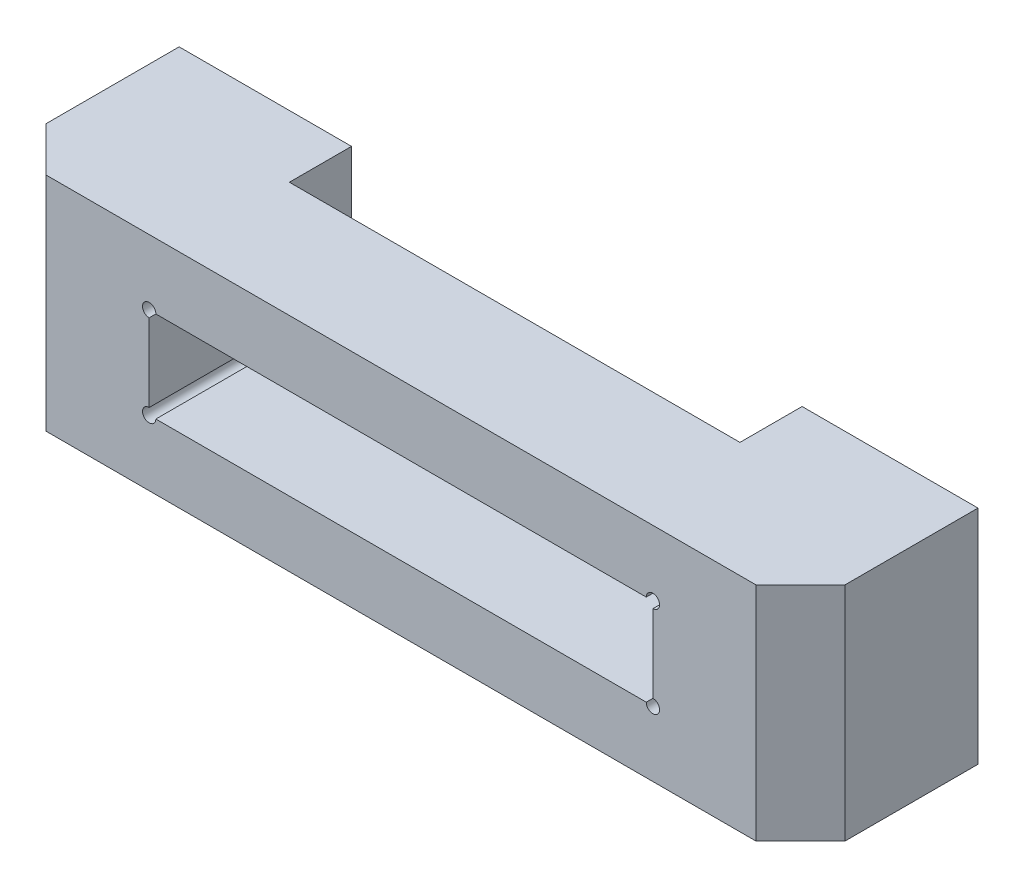
SolidWorks part; units mm, degrees
ref_plane "Front Plane" through (0, 0, 0) normal (0, 0, 1) x (1, 0, 0)
ref_plane "Top Plane" through (0, 0, 0) normal (0, 1, 0) x (1, 0, 0)
ref_plane "Right Plane" through (0, 0, 0) normal (1, 0, 0) x (0, 0, -1)
sketch "Sketch1" plane through (0, 0, 0) normal (0, 0, 1) x (1, 0, 0)
  line L0 (-90, 25) -> (90, -25) construction
  line L1 (-90, 25) -> (90, 25)
  line L2 (-90, 25) -> (-90, -25)
  line L3 (-90, -25) -> (90, -25)
  line L4 (90, 25) -> (90, -25)
  dimension "D1" = 180
  dimension "D2" = 50
extrude "Boss-Extrude1" add sketch "Sketch1" along normal blind 40
sketch "Sketch2" plane through (0, 0, 40) normal (0, 0, 1) x (1, 0, 0)
  line L1 (-56.75, 10.25) -> (56.75, 10.25)
  line L2 (-56.75, 10.25) -> (-56.75, -10.25)
  line L3 (-56.75, -10.25) -> (56.75, -10.25)
  line L4 (56.75, 10.25) -> (56.75, -10.25)
  line L5 (-56.75, 10.25) -> (56.75, -10.25) construction
  line L6 (-56.75, -10.25) -> (56.75, 10.25) construction
  point P0 (0, 0)
  dimension "D1" = 113.5
  dimension "D2" = 20.5
extrude "Cut-Extrude1" cut sketch "Sketch2" against normal through all
sketch "Sketch3" plane through (0, 0, 40) normal (0, 0, 1) x (1, 0, 0)
  circle A0 centre (-56.75, 10.25) radius 1.5
  circle A1 centre (-56.75, -10.25) radius 1.5
  circle A2 centre (56.75, 10.25) radius 1.5
  circle A3 centre (56.75, -10.25) radius 1.5
  dimension "D1" = 3
extrude "Cut-Extrude2" cut sketch "Sketch3" against normal through all
sketch "Sketch4" plane through (0, 25, 0) normal (0, 1, 0) x (1, 0, 0)
  line L0 (90, 0) -> (-90, 0) construction
  line L1 (50.3635, 0) -> (-51.1604, 0)
  line L2 (50.3635, 0) -> (50.3635, -14)
  line L3 (50.3635, -14) -> (-51.1604, -14)
  line L4 (-51.1604, 0) -> (-51.1604, -14)
  dimension "D1" = 14
extrude "Cut-Extrude3" cut sketch "Sketch4" against normal blind 30
sketch "Sketch5" plane through (0, 0, 0) normal (0, 0, -1) x (-1, 0, 0)
  line L0 (90, -25) -> (-90, -25) construction
  line L1 (56.75, -25) -> (-56.75, -25)
  line L2 (56.75, -25) -> (56.75, -10.25)
  line L3 (56.75, -10.25) -> (-56.75, -10.25)
  line L4 (-56.75, -25) -> (-56.75, -10.25)
  line L5 (55.25, -10.25) -> (-55.25, -10.25) construction
  line L6 (-56.75, -8.75) -> (-56.75, 8.75) construction
  line L7 (56.75, 8.75) -> (56.75, -8.75) construction
extrude "Cut-Extrude4" cut sketch "Sketch5" against normal blind 14
chamfer "Chamfer1" distance 10 angle 45 2 edges at (-90, 0, 40) (90, 0, 40)
